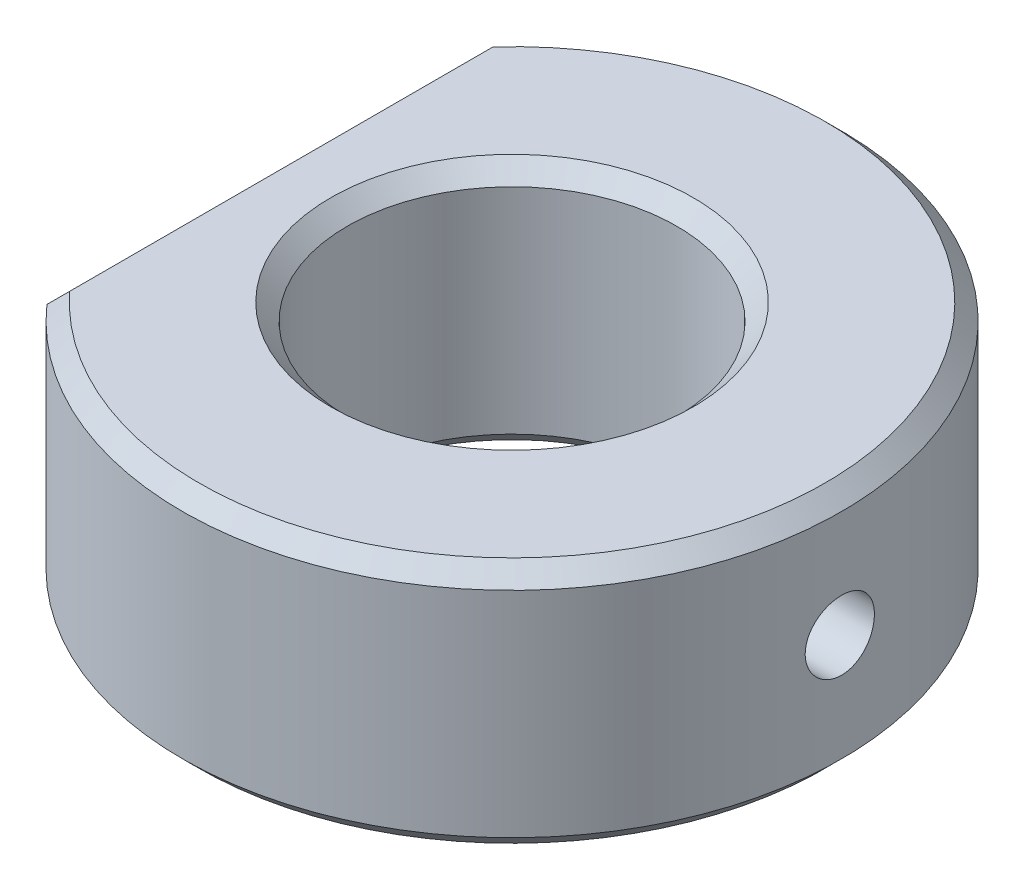
SolidWorks part; units mm, degrees
material "45号钢"
ref_plane "Front" through (0, 0, 0) normal (0, 0, 1) x (1, 0, 0)
ref_plane "Top" through (0, 0, 0) normal (0, 1, 0) x (1, 0, 0)
ref_plane "Right" through (0, 0, 0) normal (1, 0, 0) x (0, 0, -1)
sketch "草图1" plane through (0, 0, 0) normal (0, 1, 0) x (1, 0, 0)
  circle A0 centre (0, 0) radius 20
  circle A1 centre (0, 0) radius 10
  dimension "D1" = 20
  dimension "D2" = 40
extrude "凸台-拉伸1" add sketch "草图1" along normal blind 15
sketch "草图2" plane through (0, 15, 0) normal (0, 1, 0) x (1, 0, 0)
  line L1 (-24.0463, 23.8181) -> (-15, 23.8181)
  line L2 (-24.0463, 23.8181) -> (-24.0463, -15.1357)
  line L3 (-24.0463, -15.1357) -> (-15, -15.1357)
  line L4 (-15, 23.8181) -> (-15, -15.1357)
  line L5 (-24.0463, 23.8181) -> (-15, -15.1357) construction
  line L6 (-24.0463, -15.1357) -> (-15, 23.8181) construction
  circle A0 centre (0, 0) radius 20 construction
  point P0 (-19.5232, 4.3412)
  dimension "D1" = 15
extrude "切除-拉伸1" cut sketch "草图2" against normal through all
chamfer "倒角1" distance 1 angle 45 6 edges at (0, 0, 10) (0, 15, 10) (-15, 0, 0) (20, 0, 0) (-15, 15, 0) (20, 15, 0)
hole_wizard "M5 螺纹孔1" positions "草图4" profile "草图3" tap size "M5" standard "Iso"
sketch "草图4" plane through (0, 0, 0) normal (1, 0, 0) x (0, 0, -1)
  line L0 (0, 0) -> (0, 7.5) construction
  line L1 (-19, 0) -> (19, 0) construction
  point P0 (0, 7.5)
  dimension "D1" = 7.5
cosmetic thread "孔螺蚊线1" parameters "D2"=5
sketch "草图3" plane through (0, 7.5, 0) normal (0, 1, 0) x (0, 0, 1)
  line L0 (0, 0) -> (0, 20)
  line L1 (0, 20) -> (2.1, 20)
  line L2 (2.1, 20) -> (2.1, 0)
  line L5 (2.1, 0) -> (0, 0)
  line L11 (0, -6.35) -> (0, 107.95) construction
  dimension "通孔螺纹孔钻头直径" = 4.2
  dimension "通孔螺纹孔钻头深度" = 20
